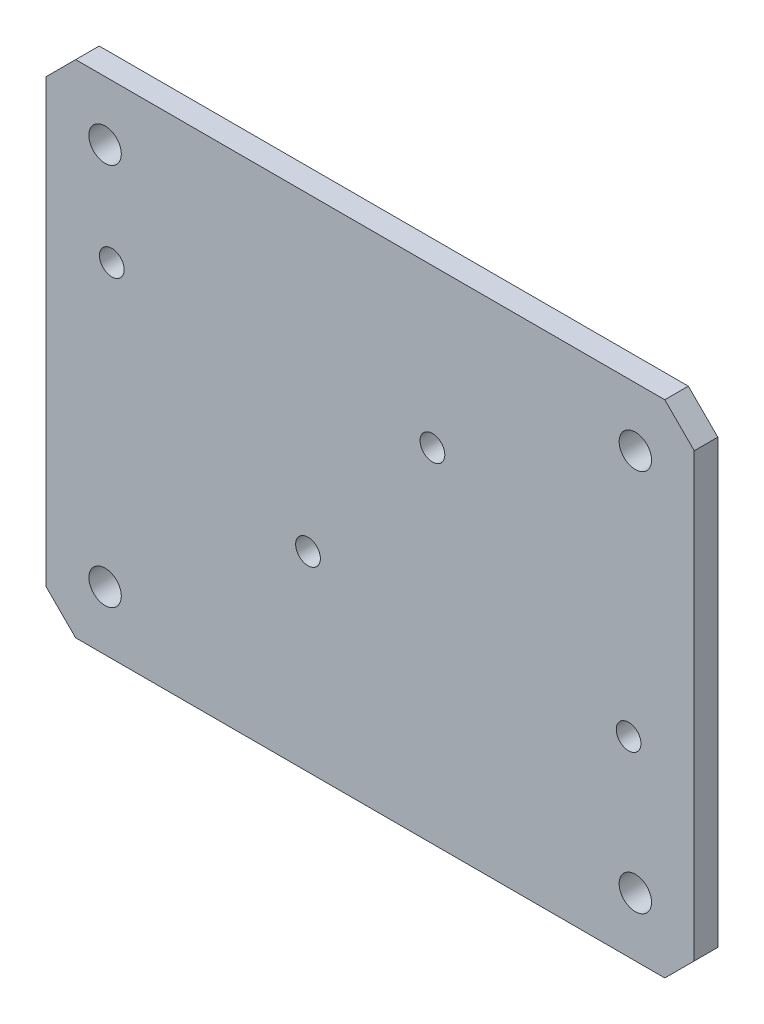
SolidWorks part; units mm, degrees
material "AL6061"
ref_plane "主视基准图" through (0, 0, 0) normal (0, 0, 1) x (1, 0, 0)
ref_plane "上视基准图" through (0, 0, 0) normal (0, 1, 0) x (1, 0, 0)
ref_plane "右视基准图" through (0, 0, 0) normal (1, 0, 0) x (0, 0, -1)
sketch "草图1" plane through (0, 0, 0) normal (0, 0, 1) x (1, 0, 0)
  line L0 (-55, 42.5) -> (55, 42.5)
  line L1 (-55, 42.5) -> (-55, -42.5)
  line L2 (-55, -42.5) -> (55, -42.5)
  line L3 (55, 42.5) -> (55, -42.5)
  line L4 (0, 42.5) -> (0, -42.5) construction
  line L5 (-55, 0) -> (55, 0) construction
  circle A0 centre (-30, -6.5) radius 4 construction
  circle A1 centre (-40, -27.5) radius 2.5 construction
  circle A2 centre (49, -35.5) radius 2.5 construction
  circle A3 centre (35, 27.5) radius 2.5 construction
  circle A4 centre (-48, 35.5) radius 2.5 construction
  dimension "D5" = 8
  dimension "D6" = 5
  dimension "D1" = 85
  dimension "D2" = 110
  dimension "D3" = 36
  dimension "D4" = 25
  dimension "D7" = 15
  dimension "D8" = 15
  dimension "D9" = 6
  dimension "D10" = 7
  dimension "D11" = 20
  dimension "D12" = 15
  dimension "D13" = 7
  dimension "D14" = 7
extrude "凸台-拉伸1" add sketch "草图1" along normal mid plane 4
chamfer "倒角1" distance 5 angle 45 4 edges at (-55, 42.5, 0) (55, 42.5, 0) (55, -42.5, 0) (-55, -42.5, 0)
hole_wizard "Ø5.5 (5.5) 直径孔1" positions "草图3" profile "草图2" hole size "Ø5.5" standard "Ansi Metric"
sketch "草图3" plane through (0, 0, 2) normal (0, 0, 1) x (1, 0, 0)
  line L0 (-50, -42.5) -> (50, -42.5) construction
  line L1 (55, -37.5) -> (55, 37.5) construction
  point P0 (45, 32.5)
  point P3 (45, -32.5)
  point P6 (-45, -32.5)
  point P9 (-45, 32.5)
  dimension "D1" = 10
  dimension "D2" = 65
  dimension "D3" = 10
  dimension "D4" = 90
sketch "草图2" plane through (45, 32.5, 2) normal (1, 0, 0) x (0, -1, 0)
  line L0 (0, 0) -> (0, 17.1977)
  line L1 (0, 17.1977) -> (2.75, 15.61)
  line L2 (2.75, 15.61) -> (2.75, 0)
  line L5 (2.75, 0) -> (0, 0)
  line L10 (0, 17.1977) -> (-2.75, 15.61) construction
  line L11 (0, -6.35) -> (0, 107.95) construction
  dimension "孔直径" = 5.5
  dimension "孔深度" = 15.61
  dimension "导头角度" = 120
sketch "草图6" plane through (0, 0, 2) normal (0, 0, 1) x (1, 0, 0)
  point P0 (10.175, 25.0525)
  point P1 (-44.245, 25.0525)
  point P3 (-10.17, -25.0525)
  point P5 (44.25, -25.0525)
hole_wizard "M5 螺纹孔3" positions "草图8" profile "草图7" tap size "M5" standard "Gb" end condition through all
sketch "草图8" plane through (0, 0, 2) normal (0, 0, 1) x (1, 0, 0)
  line L0 (-55, 2.8276) -> (55, 2.8276) construction
  line L1 (-55, 37.5) -> (-55, -37.5) construction
  line L2 (55, -37.5) -> (55, 37.5) construction
  line L5 (0, 42.5) -> (0, -42.5) construction
  line L6 (50, 42.5) -> (-50, 42.5) construction
  line L7 (-50, -42.5) -> (50, -42.5) construction
  point P0 (-43.86, 15.7326)
  point P3 (10.56, 15.7326)
  point P6 (-10.56, -10.0774)
  point P9 (43.86, -10.0774)
  dimension "D1" = 54.42
  dimension "D2" = 54.42
  dimension "D3" = 25.81
  dimension "D4" = 33.3
  dimension "D5" = 12.905
  dimension "D6" = 43.86
sketch "草图7" plane through (-43.86, 15.7326, 2) normal (1, 0, 0) x (0, -1, 0)
  line L0 (0, 0) -> (0, 4)
  line L1 (0, 4) -> (2.1, 4)
  line L2 (2.1, 4) -> (2.1, 0)
  line L5 (2.1, 0) -> (0, 0)
  line L11 (0, -6.35) -> (0, 107.95) construction
  dimension "通孔螺纹孔钻头直径" = 4.2
  dimension "通孔螺纹孔钻头深度" = 4
cosmetic thread "孔螺蚊线6" parameters "D2"=5
cosmetic thread "孔螺蚊线7" parameters "D2"=5
cosmetic thread "孔螺蚊线8" parameters "D2"=5
cosmetic thread "孔螺蚊线9" parameters "D2"=5
